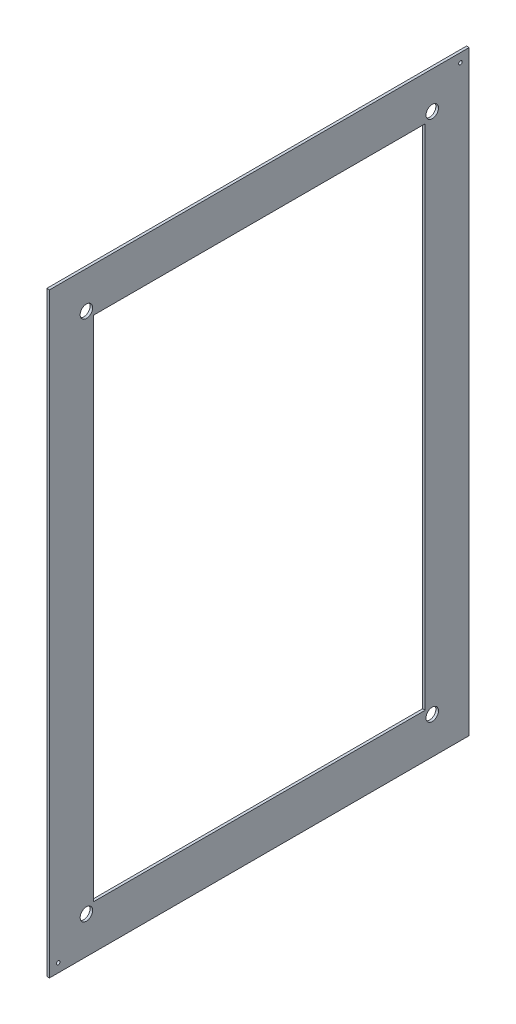
from build123d import *

# Parameters (mm, degrees)
SKETCH_1_W      = 238.5
SKETCH_1_H      = 338.6
SKETCH_1_R      = 1
SKETCH_1_R_2    = 3.55
SKETCH_1_W_2    = 188.5
SKETCH_1_H_2    = 288.6
EXTRUDE_1_DEPTH = 1.5


with BuildPart() as part:
    # 草图1 → 凸台-拉伸1 (new body)
    with BuildSketch(Plane(origin=(2615.929548806, 0, 0), x_dir=(0, 0, -1), z_dir=(1, 0, 0))):
        with Locations((-190.894615796, 1211)):
            Rectangle(SKETCH_1_W, SKETCH_1_H)
        with Locations(Location((-305.144615796, 1046.7, 0), (0, 0, 180))):
            Circle(SKETCH_1_R, mode=Mode.SUBTRACT)
        with Locations(Location((-76.644615796, 1375.3, 0), (0, 0, 180))):
            Circle(SKETCH_1_R, mode=Mode.SUBTRACT)
        with Locations(Location((-289.144615796, 1062.7, 0), (0, 0, 180))):
            Circle(SKETCH_1_R_2, mode=Mode.SUBTRACT)
        with Locations(Location((-92.644615796, 1359.3, 0), (0, 0, 180))):
            Circle(SKETCH_1_R_2, mode=Mode.SUBTRACT)
        with Locations(Location((-92.644615796, 1062.7, 0), (0, 0, 180))):
            Circle(SKETCH_1_R_2, mode=Mode.SUBTRACT)
        with Locations(Location((-289.144615796, 1359.3, 0), (0, 0, 180))):
            Circle(SKETCH_1_R_2, mode=Mode.SUBTRACT)
        with Locations((-190.894615796, 1211)):
            Rectangle(SKETCH_1_W_2, SKETCH_1_H_2, mode=Mode.SUBTRACT)
    extrude(amount=-EXTRUDE_1_DEPTH)


solid = part.part
